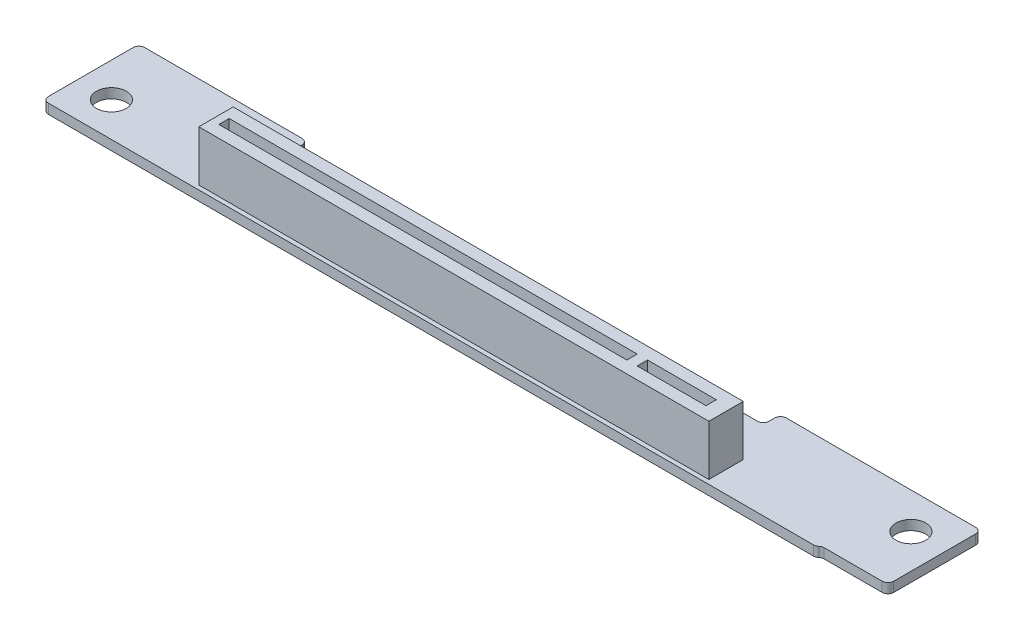
from build123d import *

# Parameters (mm, degrees)
SKETCH_2_4_R        = 2.6035
SKETCH_2_4_W        = 96.195388
SKETCH_2_4_H        = 6.300216
BOSS_EXTRUDE2_DEPTH = 1.7
SKETCH_2_4_2_W      = 96.195388
SKETCH_2_4_2_H      = 6.300216
BOSS_EXTRUDE3_DEPTH = 10.5
SKETCH4_W           = 3.597592
SKETCH4_H           = 6.300216
SKETCH4_W_2         = 3.597836
CUT_EXTRUDE1_DEPTH  = 8.8
SKETCH3_W           = 71.2
SKETCH3_H           = 2.100216
SKETCH3_W_2         = 12
SKETCH3_H_2         = 2.1
CUT_EXTRUDE2_DEPTH  = 8
MOVE_FACE1_BY       = 0.3
MOVE_FACE1_2_BY     = 0.3
MOVE_FACE1_3_BY     = 0.3


with BuildPart() as part:
    # Sketch 2_4 → Boss-Extrude2 (new body)
    # profile 1 of 2: a face of its own
    with BuildSketch(Plane(origin=(0, 0, 0), x_dir=(1, 0, 0), z_dir=(0, 1, 0))):
        with BuildLine():
            Line((134.543292, 0), (0.999998, 0))
            ThreePointArc((0.999998, 0), (0.292896914, 0.292896914), (0, 0.999998))
            Line((0, 0.999998), (0, 15.80007))
            ThreePointArc((0, 15.80007), (0.292907414, 16.507160586), (0.999998, 16.800068))
            Line((0.999998, 16.800068), (28.450032, 16.800068))
            ThreePointArc((28.450032, 16.800068), (29.157130586, 16.507168586), (29.45003, 15.80007))
            Line((29.45003, 15.80007), (29.45003, 14.800072))
            ThreePointArc((29.45003, 14.800072), (29.742916414, 14.092960414), (30.450028, 13.800074))
            Line((30.450028, 13.800074), (110.949994, 13.800074))
            ThreePointArc((110.949994, 13.800074), (111.657114586, 14.092951414), (111.949992, 14.800072))
            Line((111.949992, 14.800072), (111.949992, 15.80007))
            ThreePointArc((111.949992, 15.80007), (112.242900414, 16.507159586), (112.94999, 16.800068))
            Line((112.94999, 16.800068), (145.999962, 16.800068))
            ThreePointArc((145.999962, 16.800068), (146.707067586, 16.507175586), (146.99996, 15.80007))
            Line((146.99996, 15.80007), (146.99996, 1.49987))
            ThreePointArc((146.99996, 1.49987), (146.707065586, 0.792766414), (145.999962, 0.499872))
            Line((145.999962, 0.499872), (135.866124, 0.499872))
            ThreePointArc((135.866124, 0.499872), (135.512587346, 0.435316415), (135.204708, 0.249936))
            ThreePointArc((135.204708, 0.249936), (134.896826655, 0.064560877), (134.543292, 0))
        make_face()
        with Locations(Location((140.999972, 10.500106, 0), (0, 0, 270))):
            Circle(SKETCH_2_4_R, mode=Mode.SUBTRACT)
        with Locations(Location((5.999988, 5.999988, 0), (0, 0, 270))):
            Circle(SKETCH_2_4_R, mode=Mode.SUBTRACT)
        with Locations((70.999858, 3.899916)):
            Rectangle(SKETCH_2_4_W, SKETCH_2_4_H, mode=Mode.SUBTRACT)
    # profile 2 of 2: a face of its own
    with BuildSketch(Plane(origin=(0, 0, 0), x_dir=(1, 0, 0), z_dir=(0, 1, 0))):
        with Locations((70.999858, 3.899916)):
            Rectangle(SKETCH_2_4_W, SKETCH_2_4_H)
    extrude(amount=BOSS_EXTRUDE2_DEPTH)

    # Sketch 2_4 2 → Boss-Extrude3 (add)
    with BuildSketch(Plane(origin=(0, 0, 0), x_dir=(1, 0, 0), z_dir=(0, 1, 0))):
        with Locations((70.999858, 3.899916)):
            Rectangle(SKETCH_2_4_2_W, SKETCH_2_4_2_H)
    extrude(amount=BOSS_EXTRUDE3_DEPTH)

    # Sketch4 → Cut-Extrude1 (cut)
    with BuildSketch(Plane(origin=(0, 10.5, 0), x_dir=(1, 0, 0), z_dir=(0, 1, 0))):
        with Locations((117.298756, 3.899916)):
            Rectangle(SKETCH4_W, SKETCH4_H)
        with Locations((24.701082, 3.899916)):
            Rectangle(SKETCH4_W_2, SKETCH4_H)
    extrude(amount=-CUT_EXTRUDE1_DEPTH, mode=Mode.SUBTRACT)

    # Sketch3 → Cut-Extrude2 (cut)
    with BuildSketch(Plane(origin=(0, 10.5, 0), x_dir=(1, 0, 0), z_dir=(0, 1, 0))):
        with Locations((63.5, 3.899916)):
            Rectangle(SKETCH3_W, SKETCH3_H)
        with Locations((106.9, 3.899808)):
            Rectangle(SKETCH3_W_2, SKETCH3_H_2)
    extrude(amount=-CUT_EXTRUDE2_DEPTH, mode=Mode.SUBTRACT)

    # Move Face1: a face moved outward by 0.3
    extrude(part.faces().sort_by_distance((63.5, 6.5, -4.950024))[0], amount=MOVE_FACE1_BY, dir=(0, 0, 1))

    # Move Face1 2: a face moved inward by 0.3
    extrude(part.faces().sort_by_distance((70.99998, 6.1, -7.050024))[0], amount=MOVE_FACE1_2_BY, dir=(0, 0, 1), mode=Mode.SUBTRACT)

    # Move Face1 3: a face moved outward by 0.3
    extrude(part.faces().sort_by_distance((106.9, 6.5, -4.949808))[0], amount=MOVE_FACE1_3_BY, dir=(0, 0, 1))


solid = part.part
